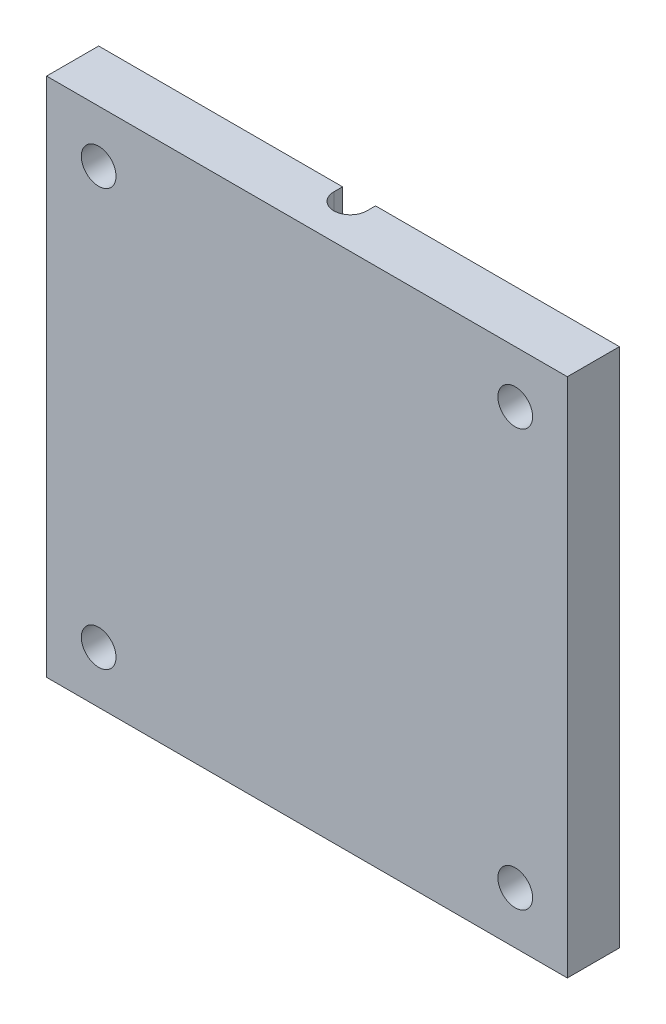
SolidWorks part; units mm, degrees
ref_plane "Front Plane" through (0, 0, 0) normal (0, 0, 1) x (1, 0, 0)
ref_plane "Top Plane" through (0, 0, 0) normal (0, 1, 0) x (1, 0, 0)
ref_plane "Right Plane" through (0, 0, 0) normal (1, 0, 0) x (0, 0, -1)
sketch "Sketch1" plane through (0, 0, 0) normal (0, 0, 1) x (1, 0, 0)
  line L1 (-15, -15) -> (15, -15)
  line L2 (-15, -15) -> (-15, 15)
  line L3 (-15, 15) -> (15, 15)
  line L4 (15, -15) -> (15, 15)
  line L5 (-15, -15) -> (15, 15) construction
  line L6 (-15, 15) -> (15, -15) construction
  point P0 (0, 0)
  dimension "D1" = 30
  dimension "D2" = 30
extrude "Boss-Extrude1" add sketch "Sketch1" along normal blind 3
sketch "Sketch2" plane through (0, 0, 3) normal (0, 0, 1) x (1, 0, 0)
  line L5 (-12, -12) -> (12, 12) construction
  line L6 (-12, 12) -> (12, -12) construction
  circle A0 centre (-12, 12) radius 1
  circle A1 centre (12, 12) radius 1
  circle A5 centre (12, -12) radius 1
  circle A6 centre (-12, -12) radius 1
  circle A7 centre (12, 12) radius 1 [skipped]
  point P0 (0, 0)
  point P19 (0, 0)
  dimension "D4" = 2
  dimension "D5" = 2
  dimension "D1" = 24
  dimension "D2" = 24
  dimension "D3" = 4
extrude "Cut-Extrude1" cut sketch "Sketch2" against normal blind 19
sketch "Sketch3" plane through (0, -15, 0) normal (0, -1, 0) x (1, 0, 0)
  line L1 (-15, 3) -> (-15, 0) construction
  line L2 (-15, 0) -> (15, 0) construction
  line L3 (0.95, 0.5) -> (0.95, 0)
  line L4 (-0.95, 0) -> (0.95, 0)
  line L5 (-0.95, 0) -> (-0.95, 0.5)
  arc A1 (0.95, 0.5) -> (-0.95, 0.5) centre (0, 0.5) ccw
  dimension "D1" = 15
  dimension "D3" = 0.95
  dimension "D2" = 0.5
extrude "Cut-Extrude2" cut sketch "Sketch3" against normal blind 42
